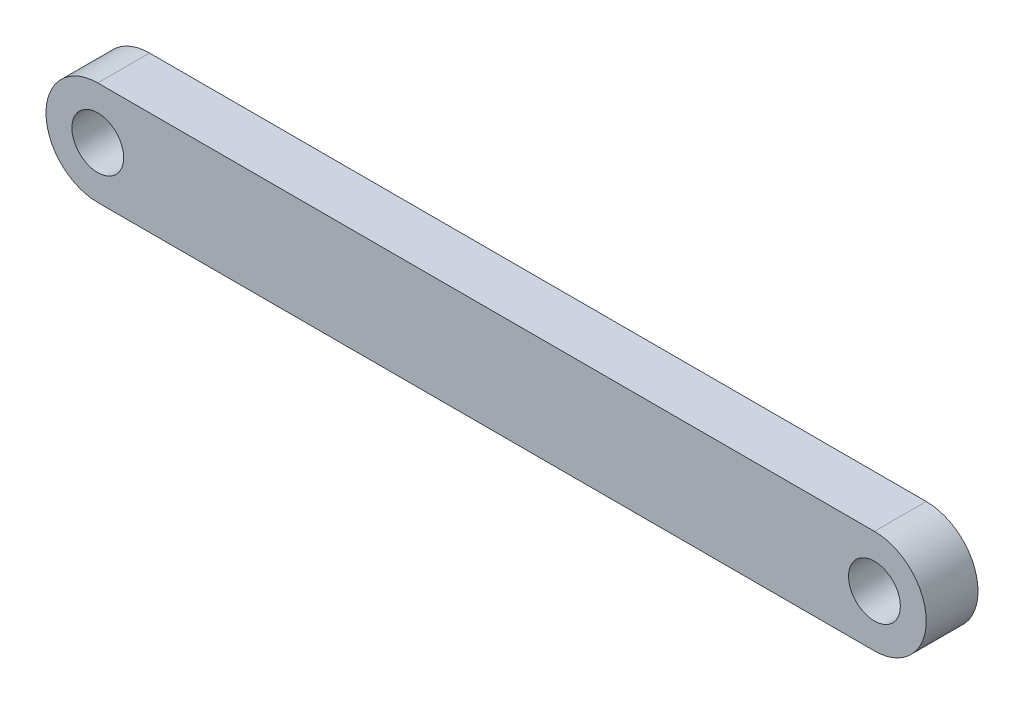
from build123d import *

# Parameters (mm, degrees)
SKETCH1_R           = 1.5
BOSS_EXTRUDE1_DEPTH = 3


with BuildPart() as part:
    # Sketch1 → Boss-Extrude1 (new body)
    with BuildSketch(Plane.XY):
        with BuildLine():
            Line((0, 3), (45, 3))
            ThreePointArc((45, 3), (48, 0), (45, -3))
            Line((45, -3), (0, -3))
            ThreePointArc((0, -3), (-3, 0), (0, 3))
        make_face()
        Circle(SKETCH1_R, mode=Mode.SUBTRACT)
        with Locations((45, 0)):
            Circle(SKETCH1_R, mode=Mode.SUBTRACT)
    extrude(amount=BOSS_EXTRUDE1_DEPTH)


solid = part.part
